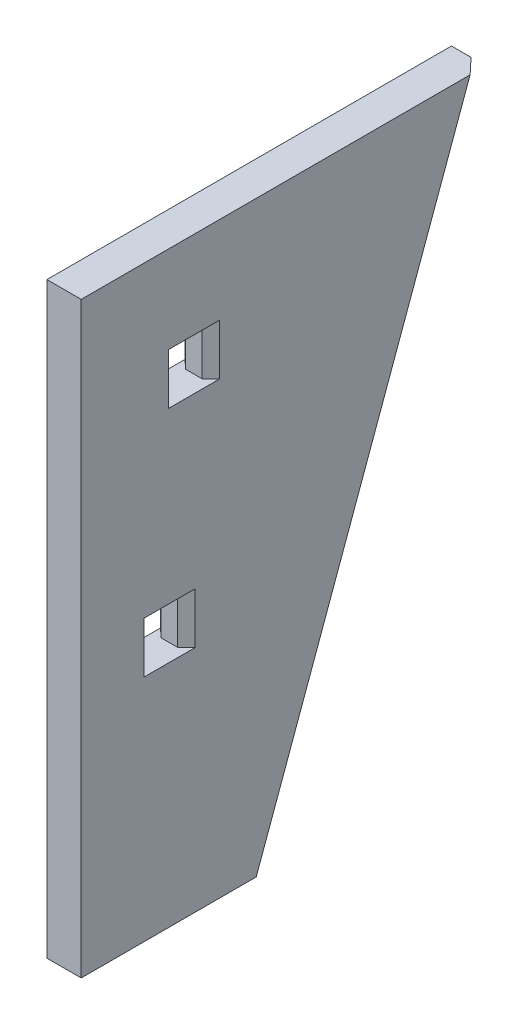
from build123d import *

# Parameters (mm, degrees)
BOSS_EXTRUDE1_DEPTH = 17.5
CUT_EXTRUDE1_START  = 185
CUT_EXTRUDE1_DEPTH  = 26
CHAMFER2_SIZE       = 15
CUT_EXTRUDE2_START  = -40
CUT_EXTRUDE2_DEPTH  = 26


with BuildPart() as part:
    # Sketch1 → Boss-Extrude1 (new, symmetric)
    with BuildSketch(Plane(origin=(0, 0, 0), x_dir=(0, 0, -1), z_dir=(1, 0, 0))):
        Polygon((0, 0), (0, 300), (413, 300), (194.61785944, -300), (0, -300), align=None)
    extrude(amount=BOSS_EXTRUDE1_DEPTH, both=True)

    # Sketch2 → Cut-Extrude1 (cut, symmetric)
    with BuildSketch(Plane(origin=(0, 0, 0), x_dir=(1, 0, 0), z_dir=(0, 1, 0)).offset(CUT_EXTRUDE1_START)):
        Polygon((-17.5, 89), (-8.5, 97.5), (8.5, 97.5), (17.5, 89), (17.5, 141), (8.5, 132.5), (-8.5, 132.5), (-17.5, 141), align=None)
    extrude(amount=CUT_EXTRUDE1_DEPTH, both=True, mode=Mode.SUBTRACT)

    # Chamfer2
    chamfer2_edges = [part.edges().sort_by_distance(p)[0] for p in [
        (17.5, 0, -303.80892972),
    ]]
    chamfer(chamfer2_edges, length=CHAMFER2_SIZE)

    # Sketch3 → Cut-Extrude2 (cut, symmetric)
    with BuildSketch(Plane(origin=(0, 0, 0), x_dir=(1, 0, 0), z_dir=(0, 1, 0)).offset(CUT_EXTRUDE2_START)):
        Polygon((-17.5, 64), (-8.5, 72.5), (8.5, 72.5), (17.5, 64), (17.5, 116), (8.5, 107.5), (-8.5, 107.5), (-17.5, 116), align=None)
    extrude(amount=CUT_EXTRUDE2_DEPTH, both=True, mode=Mode.SUBTRACT)


solid = part.part
